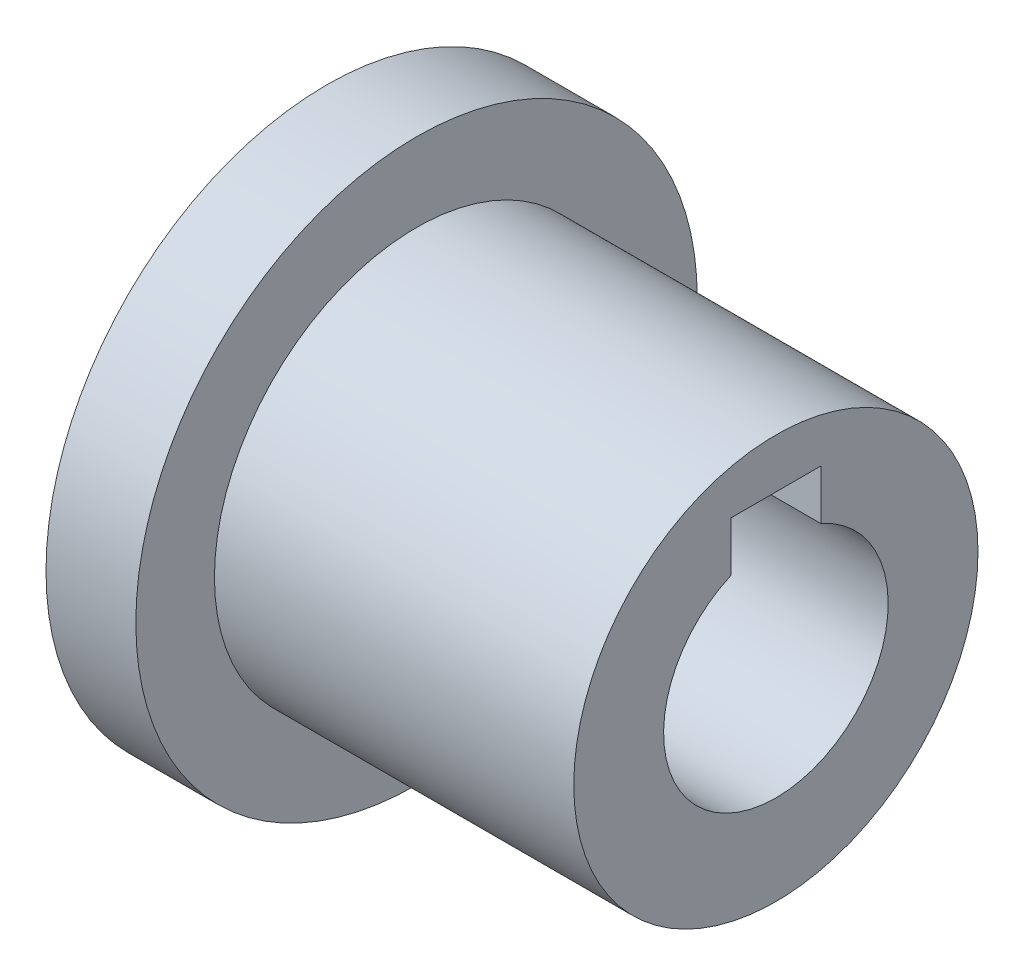
from build123d import *

# Parameters (mm, degrees)
SKETCH_2_W          = 4
SKETCH_2_H          = 6.8
CUT_EXTRUDE_1_DEPTH = 27.69269563


with BuildPart() as part:
    # 草图1 → 旋转1 (revolve)
    with BuildSketch(Plane.XY, mode=Mode.PRIVATE) as revolve_1_sk:
        Polygon((0, 5), (20, 5), (20, 9), (4, 9), (4, 12.5), (0, 12.5), align=None)
    revolve(revolve_1_sk.sketch.rotate(Axis((0, 0, 0), (1, 0, 0)), 90), axis=Axis((0, 0, 0), (1, 0, 0)))

    # 草图2 → 切除-拉伸1 (cut, through all)
    with BuildSketch(Plane.ZY):
        with Locations((0, 3.4)):
            Rectangle(SKETCH_2_W, SKETCH_2_H)
    extrude(amount=-CUT_EXTRUDE_1_DEPTH, mode=Mode.SUBTRACT)


solid = part.part
